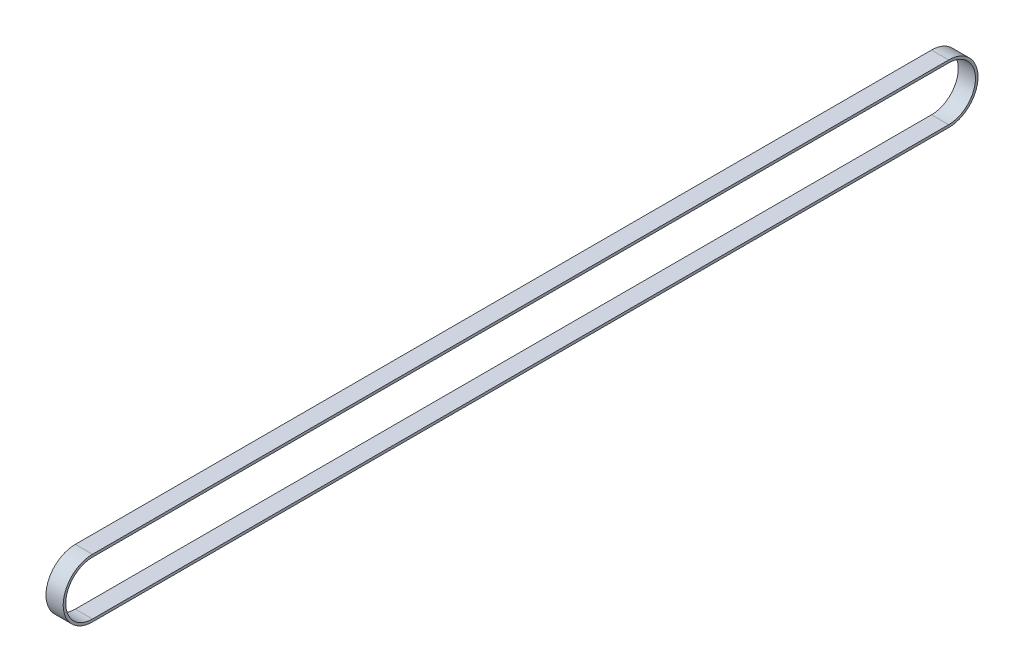
SolidWorks part; units mm, degrees
material "聚脂树脂"
ref_plane "前视基准面" through (0, 0, 0) normal (0, 0, 1) x (1, 0, 0)
ref_plane "上视基准面" through (0, 0, 0) normal (0, 1, 0) x (1, 0, 0)
ref_plane "右视基准面" through (0, 0, 0) normal (1, 0, 0) x (0, 0, -1)
sketch "草图2" plane through (0, 0, 0) normal (1, 0, 0) x (0, 0, -1)
  line L0 (0, 47.75) -> (-1496.41, 47.75)
  line L6 (-1496.41, -47.75) -> (0, -47.75)
  arc A0 (0, -47.75) -> (0, 47.75) centre (0, 0) ccw
  arc A1 (-1496.41, 47.75) -> (-1496.41, -47.75) centre (-1496.41, 0) ccw
  dimension "D2" = 95.5
  dimension "D7" = 1496.41
extrude "拉伸-薄壁1" add sketch "草图2" along normal mid plane 30 thin
